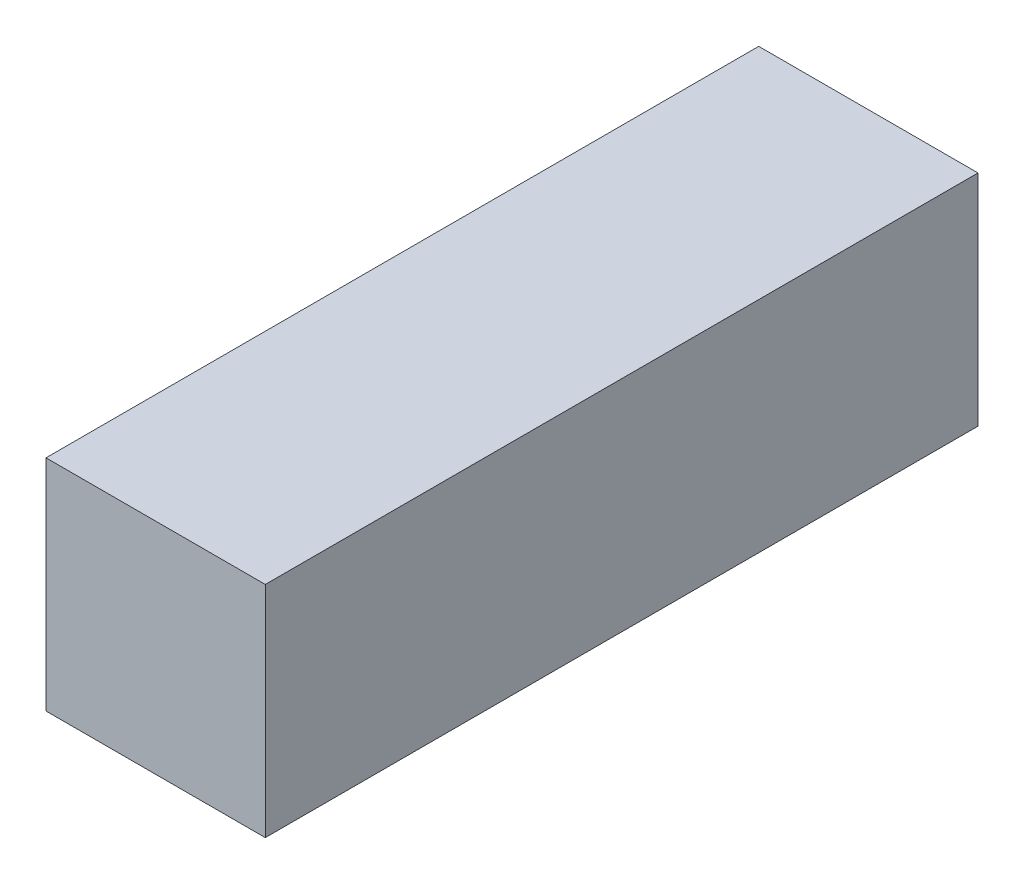
from build123d import *

# Parameters (mm, degrees)
SKETCH1_W           = 20
SKETCH1_H           = 65
BOSS_EXTRUDE1_DEPTH = 20


with BuildPart() as part:
    # Sketch1 → Boss-Extrude1 (new body)
    with BuildSketch(Plane(origin=(0, 0, 0), x_dir=(1, 0, 0), z_dir=(0, 1, 0))):
        Rectangle(SKETCH1_W, SKETCH1_H)
    extrude(amount=BOSS_EXTRUDE1_DEPTH)


solid = part.part
